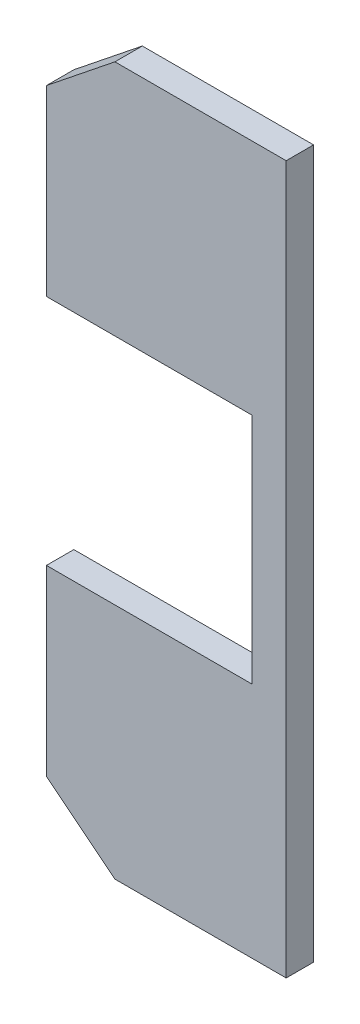
SolidWorks part; units mm, degrees
material "普通碳钢"
ref_plane "Front Plane" through (0, 0, 0) normal (0, 0, 1) x (1, 0, 0)
ref_plane "Top Plane" through (0, 0, 0) normal (0, 1, 0) x (1, 0, 0)
ref_plane "Right Plane" through (0, 0, 0) normal (1, 0, 0) x (0, 0, -1)
sketch "Sketch1" plane through (0, 0, 0) normal (0, 0, 1) x (1, 0, 0)
  line L0 (-7.5, 155) -> (-7.5, -155)
  line L1 (-7.5, -155) -> (7.5, -155)
  line L2 (7.5, -155) -> (7.5, 155)
  line L3 (7.5, 155) -> (-7.5, 155)
  point P2 (-7.5, 0)
  point P5 (0, 155)
  dimension "D1" = 15
  dimension "D2" = 310
extrude "Extrude1" add sketch "Sketch1" along normal mid plane 12
sketch "Sketch3" plane through (0, 0, 0) normal (0, 0, 1) x (1, 0, 0)
  line L0 (0, 0) -> (-156.1525, 0) construction
  line L1 (-7.5, 155) -> (-67.5, 155)
  line L2 (-67.5, 155) -> (-97.5, 131)
  line L3 (-97.5, 131) -> (-97.5, 51)
  line L4 (-97.5, 51) -> (-7.5, 51)
  line L5 (-7.5, 155) -> (-7.5, -155) construction
  line L6 (-7.5, 51) -> (-7.5, 155)
  line L7 (-7.5, -51) -> (-7.5, -155)
  line L8 (-97.5, -51) -> (-7.5, -51)
  line L9 (-97.5, -131) -> (-97.5, -51)
  line L10 (-67.5, -155) -> (-97.5, -131)
  line L11 (-7.5, -155) -> (-67.5, -155)
  dimension "D1" = 51
  dimension "D2" = 90
  dimension "D3" = 60
  dimension "D4" = 80
extrude "Extrude3" add sketch "Sketch3" along normal mid plane 12
